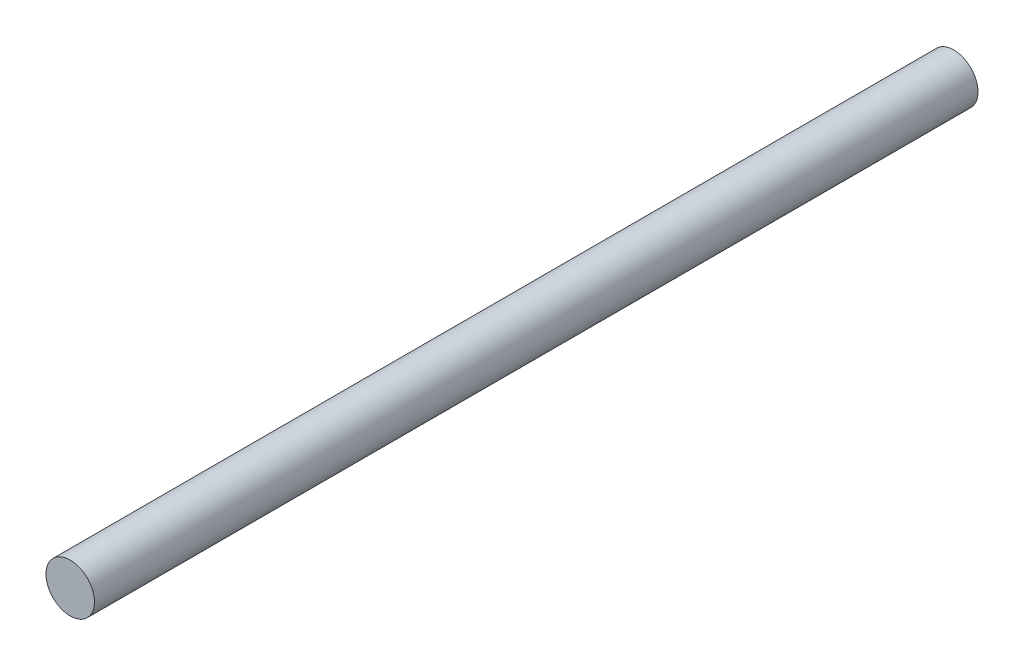
SolidWorks part; units mm, degrees
material "SWRM3"
ref_plane "Front Plane" through (0, 0, 0) normal (0, 0, 1) x (1, 0, 0)
ref_plane "Top Plane" through (0, 0, 0) normal (0, 1, 0) x (1, 0, 0)
ref_plane "Right Plane" through (0, 0, 0) normal (1, 0, 0) x (0, 0, -1)
sketch "Sketch1" plane through (0, 0, 0) normal (0, 0, 1) x (1, 0, 0)
  circle A0 centre (-35, 4.7) radius 2.8
  dimension "D1" = 5.6
extrude "Boss-Extrude1" add sketch "Sketch1" against normal blind 102
